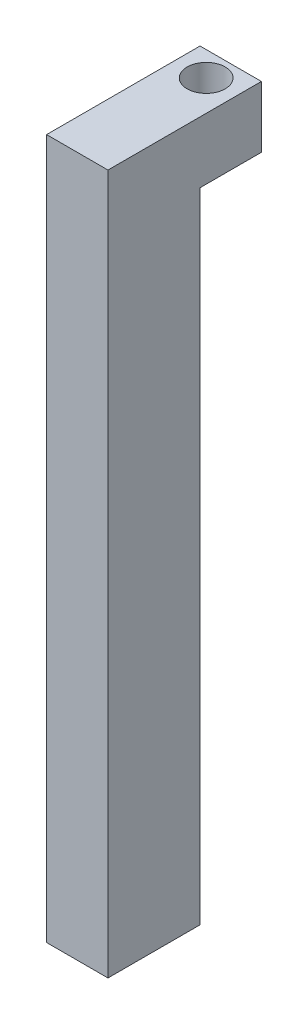
SolidWorks part; units mm, degrees
ref_plane "Front Plane" through (0, 0, 0) normal (0, 0, 1) x (1, 0, 0)
ref_plane "Top Plane" through (0, 0, 0) normal (0, 1, 0) x (1, 0, 0)
ref_plane "Right Plane" through (0, 0, 0) normal (1, 0, 0) x (0, 0, -1)
sketch "Sketch1" plane through (0, 0, 0) normal (0, 1, 0) x (1, 0, 0)
  line L1 (-5, -7.5) -> (5, -7.5)
  line L2 (-5, -7.5) -> (-5, 7.5)
  line L3 (-5, 7.5) -> (5, 7.5)
  line L4 (5, -7.5) -> (5, 7.5)
  line L5 (-5, -7.5) -> (5, 7.5) construction
  line L6 (-5, 7.5) -> (5, -7.5) construction
  point P0 (0, 0)
  dimension "D1" = 15
  dimension "D2" = 10
extrude "Boss-Extrude1" add sketch "Sketch1" along normal blind 114
sketch "Sketch2" plane through (0, 114, 0) normal (0, 1, 0) x (1, 0, 0)
  line L1 (-5, 7.5) -> (5, 7.5)
  line L2 (-5, 7.5) -> (-5, 17.5)
  line L3 (-5, 17.5) -> (5, 17.5)
  line L4 (5, 7.5) -> (5, 17.5)
  circle A0 centre (0, 13.5) radius 3.1
  dimension "D3" = 6.2
  dimension "D4" = 6
  dimension "D1" = 10
  dimension "D2" = 10
extrude "Boss-Extrude2" add sketch "Sketch2" against normal blind 10
hole_wizard "M4 Tapped Hole1" positions "Sketch3" profile "Sketch4" tap size "M4" standard "GB"
sketch "Sketch3" plane through (0, 0, 0) normal (0, -1, 0) x (-1, 0, 0)
  line L0 (5, -7.5) -> (-5, -7.5) construction
  line L1 (5, 7.5) -> (5, -7.5) construction
  point P0 (0, 3.5)
  point P2 (0, -3.5)
  dimension "D1" = 7
  dimension "D2" = 4
  dimension "D3" = 5
  dimension "D4" = 5
sketch "Sketch4" plane through (0, 0, -3.5) normal (1, 0, 0) x (0, 0, -1)
  line L0 (0, 0) -> (0, 12.4914)
  line L1 (0, 12.4914) -> (1.65, 11.5)
  line L2 (1.65, 11.5) -> (1.65, 0.375)
  line L3 (1.65, 0.375) -> (2.025, 0)
  line L5 (2.025, 0) -> (0, 0)
  line L6 (-1.65, 0.375) -> (-2.025, 0) construction
  line L10 (0, 12.4914) -> (-1.65, 11.5) construction
  line L11 (0, -6.35) -> (0, 107.95) construction
  dimension "螺纹孔钻头直径" = 3.3
  dimension "螺纹孔钻头深度" = 11.5
  dimension "近端锥形沉头孔直径" = 4.05
  dimension "近端锥形沉头孔角度" = 90
  dimension "导头角度" = 118
cosmetic thread "Hole thread 1" parameters "D1"=8, "D2"=4
cosmetic thread "Hole thread 2" parameters "D1"=8, "D2"=4
